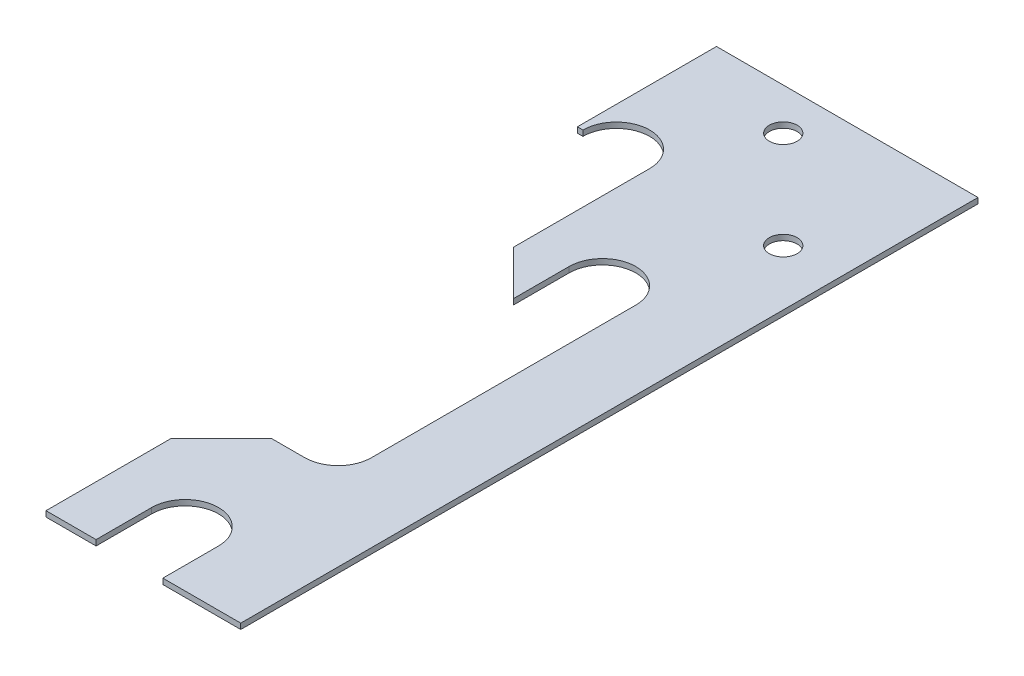
from build123d import *

# Parameters (mm, degrees)
SKETCH_1_R      = 5
EXTRUDE_1_DEPTH = 2


with BuildPart() as part:
    # 草图1 → 凸台-拉伸1 (new body)
    with BuildSketch(Plane(origin=(0, 0, 0), x_dir=(1, 0, 0), z_dir=(0, 1, 0))):
        with BuildLine():
            Line((0, 0), (0, 50))
            Line((0, 50), (94, 50))
            Line((94, 50), (94, -215))
            Line((94, -215), (66, -215))
            Line((66, -215), (66, -195))
            ThreePointArc((66, -195), (54, -183), (42, -195))
            Line((42, -195), (42, -215))
            Line((42, -215), (24, -215))
            Line((24, -215), (24, -170))
            Line((24, -170), (42, -152))
            Line((42, -152), (54, -152))
            ThreePointArc((54, -152), (62.485281374, -148.485281374), (66, -140))
            Line((66, -140), (66, -45))
            ThreePointArc((66, -45), (54, -33), (42, -45))
            Line((42, -45), (42, -65))
            Line((42, -65), (26, -49))
            Line((26, -49), (26, 0))
            ThreePointArc((26, 0), (14, 12), (2, 0))
            Line((2, 0), (0, 0))
        make_face()
        with Locations(Location((39, 35, 0), (0, 0, 90))):
            Circle(SKETCH_1_R, mode=Mode.SUBTRACT)
        with Locations(Location((74, 0, 0), (0, 0, 90))):
            Circle(SKETCH_1_R, mode=Mode.SUBTRACT)
    extrude(amount=EXTRUDE_1_DEPTH)


solid = part.part
